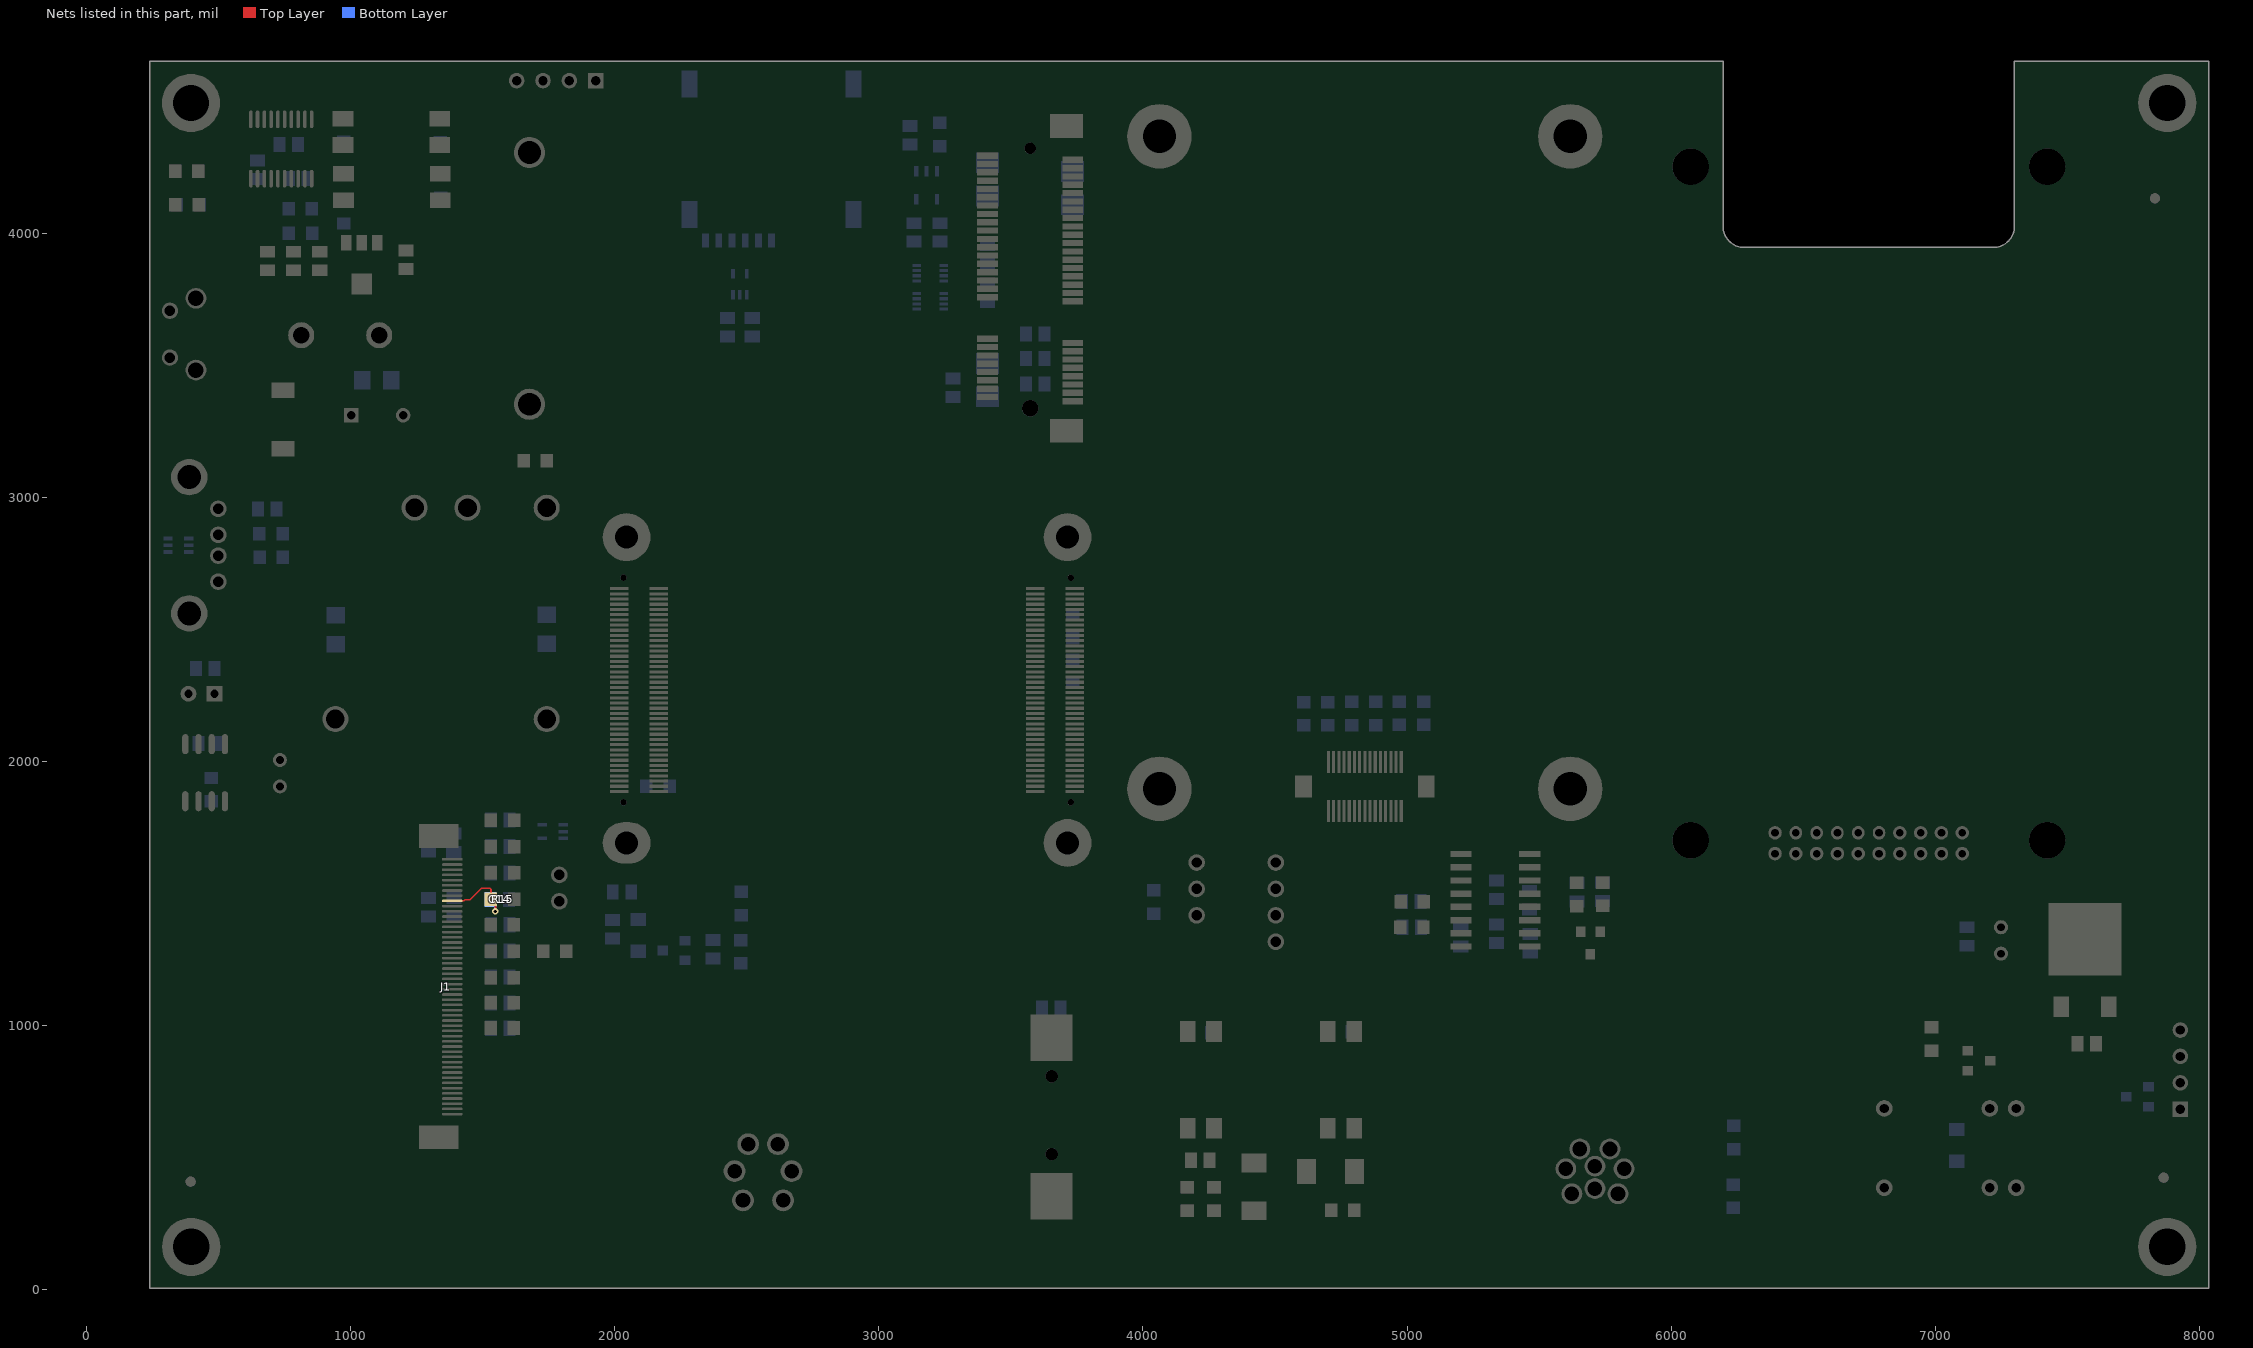
[diagram p0: the nets of this part, all layers, seen from the top]
# Altium PCB MISC82794.PcbDoc (part 5 of 5)
Units mil, origin at the board's own origin, x right, y up, seen from the top; angles counter-clockwise.
Board outline 7795.28 x 4645.67 mil, 4 copper layers (Top Layer, GND, POWER, Bottom Layer); 157 components, 133 nets, 768 pads, 456 vias.

## Via types
v1: diameter 24, hole 12, Top Layer to Bottom Layer, 258 vias
v2: diameter 40, hole 20, Top Layer to Bottom Layer, 197 vias
v3: diameter 30, hole 15, Top Layer to Bottom Layer, 1 vias

## Nets (pads, with @x,y where several pads share a name; then routed paths per layer and width w, separated by ;. In a path a pad name is that pad's centre, name@x,y a point inside that pad or via, vN(x,y) a via of type N, cw(c..) or ccw(c..) an arc to the next point about the centre after c; other vN are vias at no path point) (continued)
YP: C14.1 J1.9 R15.2 | length 313.2
  Top Layer w6: J1.9@1385.39,1472.65 1428.74,1472.65 1432.58,1476.49 1451.97,1476.49 1496.48,1521 1528,1521 1532,1517 R15.2@1532,1478.6 1549,1461.6 1549,1434 v1(1548,1433)
  Bottom Layer w6: C14.1@1531,1478.6 1547,1462.6 1547,1436 1549,1434 v1(1548,1433)
pads on no net: BT1.0 D5.1 D5.3 H1.8 H2.8 H3.8 H4.8 J1.10 J1.11 J1.13 J1.14 J1.15 J1.16 J1.18 J1.30 J1.31 J1.32 J1.40 J1.41 J1.48 J1.49 J1.50 J2.0 J2.1 J2.2 J2.3 J2.4 J2.A1 J2.A2 J2.A3 J2.A4 J2.A5 J2.A6 J2.A17 J2.A19 J2.A21 J2.A23 J2.A25 J2.A27 J2.A31 J2.A42 J2.A44 J2.A46 J2.A48 J2.A49 J2.A50 J2.A51 J2.A52 J2.A53 J2.A54 J2.A55 J2.A56 J2.A57 J2.A59 J2.A60 J2.A61 J2.A62 J2.A63 J2.A64 J2.A65 J2.A66 J2.A67 J2.A68 J2.A70 J2.A72 J2.A74 J2.A76 J2.A78 J2.A79 J2.A80 J2.B7 J2.B8 J2.B9 J2.B10 J2.B11 J2.B12 J2.B13 J2.B14 J2.B15 J2.B16 J2.B17 J2.B18 J2.B19 J2.B21 J2.B22 J2.B23 J2.B24 J2.B26 J2.B27 J2.B28 J2.B30 J2.B31 J2.B33 J2.B34 J2.B36 J2.B38 J2.B40 J2.B42 J2.B46 J2.B48 J2.B52 J2.B54 J2.B56 J2.B58 J2.B60 J2.B62 J2.B64 J2.B65 J2.B66 J2.B67 J2.B68 K1.3 K1.6 S1.3 S1.4 U6.0 U6.1 U6.3 U6.5 U6.6 U6.7 U6.11 U6.13 U6.16 U6.20 U6.23 U6.25 U6.28 U6.30 U6.31 U6.32 U6.33 U6.36 U6.38 U6.44 U6.45 U6.46 U6.47 U6.48 U6.49 U6.51 U6.53 U6.54 U9.3 U9.4 U9.7 U9.8 U9.20 U9.21 U9.22 U9.23 U9.24 U11.1 U11.2 U11.8 U13.1 U13.2 U13.3 U13.5 U13.6 U13.11 U13.12 U13.16 U13.17 U13.19 U13.20 U15.6 U15.10 U15.11 U17.0 U17.2 U17.4 U17.6 U17.8 U17.10 U17.12 U17.13 U17.15 U17.16 U17.17 U17.29 U17.31 U19.3 U19.6

## Polygon pours and split planes (outlines as drawn)
USB0_VBUS_5V on Bottom Layer "Top Layer-No Net" (solid, remove dead copper, pour order 1000): 1935.12,1937 1935.12,1914.88 1945,1905 1948,1902 1963,1902 1973,1902 1980,1909 1981,1910 1981,1925 1981,1934 1970,1945 1949,1945 1942.64,1945 1934.64,1937
VDD_12V on Bottom Layer "Top Layer-No Net" (solid, remove dead copper, pour order 1001): 4056,310.7 4056,257.46 4061,251.55 4064,248 4096,248 4189.74,248 4194,253.04 4198,257.77 4198,291.77 4198,321.35 4190,330.82 4189,332 4111,332 4067,332 4062,326.08 4056,318.99 4056,310.7
VDD_5V on Bottom Layer "Top Layer-No Net" (solid, remove dead copper, pour order 1002): 1239,1654 1239,1594 1248,1585 1253,1580 1274,1580 1311,1580 1321,1590 1362,1631 1390,1631 1416.66,1631 1420.66,1635 1425,1639.34 1425,1647 1425,1677.66 1420.66,1682 1419.66,1683 1412,1683 1244,1683 1239,1678 1239,1654
VDD_3.3 on Bottom Layer "Top Layer-No Net" (solid, remove dead copper, pour order 1003): 3075,4339 3075,4235 3091,4219 3097,4213 3131,4213 3150,4213 3153,4216 3156,4219 3156,4245 3156,4353 3150,4359 3148,4361 3128,4361 3082,4361 3075,4354 3075,4338
VDD_3.3 on Bottom Layer "Top Layer-No Net" (solid, remove dead copper, pour order 1004): 1237,1556 1237,1478 1249,1466 1256,1459 1278,1459 1424,1459 1428,1463 1431,1466 1431,1487 1431,1543 1405,1569 1401,1573 1309,1573 1246,1573 1237,1564 1237,1556
VDD_3.3 on Bottom Layer "Top Layer-No Net" (solid, remove dead copper, pour order 1005): 2895,1926 2895,1893 2901,1887 2907,1881 2928,1881 2932,1881 2934,1883 2936,1885 2936,1901 2936,1933 2933,1936 2931,1938 2924,1938 2902,1938 2898,1934 2895,1931 2895,1926
GND1 on Bottom Layer "Top Layer-No Net" (solid, remove dead copper, pour order 1006): 6200,638 6200,599 6204,595 6205,594 6240,594 6340,594 6348,602 6348,625 6348,656 6341,663 6335,669 6304,669 6207,669 6201,663 6200,662 6200,638
GND1 on Bottom Layer "Top Layer-No Net" (solid, remove dead copper, pour order 1007): 4227.2,303.17 4227.2,234.61 4234.4,229.37 4240.4,225 4270.4,225 4304,225 4312.4,231.12 4316,233.74 4316,259.96 4316,320.61 4309.28,325.5 4304.48,329 4281.2,329 4235.6,329 4228.4,323.76 4226,322.01 4226,303.17
GND on Bottom Layer "Top Layer-No Net" (solid, remove dead copper, pour order 1008): 61.25,4802.36 61.25,-271.65 -22.75,-355.65 228.25,-104.65 8117.25,-104.65 8117.25,4836.36 8251.25,4970.36 8132.25,4851.36 88.25,4851.36 88.25,4831.36 65.25,4808.36
GND1 on Top Layer "Top Layer-No Net" (solid, remove dead copper): 653,3873 653,3829 710,3772 750,3732 847,3732 903,3732 939,3696 943,3692 943,3650 943,3604 973,3574 993,3554 1074,3554 1097,3531 1149,3479 1149,3360 1149,3268 1159,3258 1166,3251 1190,3251 1276,3251 1288,3263 1295,3270 1295,3331 1295,3867 1276,3886 1273,3889 1244,3889 1082,3889 1075,3896 1069,3902 1069,3934 1069,3987 1062,3994 1059,3997 1051,3997 1023,3997 1021,3995 1019,3993 1019,3986 1019,3903 1015,3899 1002,3886 917,3886 659,3886 653,3880 653,3873
VDD_12V on Top Layer "Top Layer-No Net" (solid, remove dead copper): 268.85,3562.15 268.85,3508.15 268.85,3505.15 279.85,3494.15 334.85,3494.15 335.85,3494.15 390.85,3549.15 482.85,3549.15 509.85,3522.15 509.85,3508.15 509.85,3410.15 563.85,3356.15 778.85,3356.15 779.85,3356.15 890.85,3245.15 1023.85,3245.15 1041.85,3263.15 1042.85,3264.15 1042.85,3440.15 883.85,3599.15 883.85,3606.15 883.85,3664.15 836.85,3711.15 748.85,3711.15 743.85,3716.15 632.85,3827.15 632.85,3881.15 632.85,3894.15 640.85,3902.15 644.85,3906.15 671.85,3906.15 991.85,3906.15 1003.85,3918.15 1003.85,3942.15 1003.85,3997.15 999.85,4001.15 952.85,4001.15 793.85,4001.15 775.85,3983.15 760.85,3968.15 713.85,3968.15 568.85,3968.15 544.85,3944.15 527.85,3927.15 527.85,3906.15 527.85,3730.15 431.85,3634.15 429.85,3632.15 343.85,3632.15 324.85,3632.15 276.85,3584.15 268.85,3576.15 268.85,3562.15
USB0_VBUS_5V on Top Layer "Top Layer-No Net" (solid, remove dead copper, pour order 1009): 1935.12,1933 1935.12,1910.88 1940,1906 1946,1900 1960,1900 1968,1900 1979,1911 1986,1918 1995,1918 2055,1918 2056,1919 2057,1920 2057,1923 2057,1932 2055,1934 2054,1935 2049,1935 1977,1935 1970,1942 1967,1945 1957,1945 1942,1945 1938,1941 1935.12,1938.12 1935.12,1933
NetC4_1 on Top Layer "Top Layer-No Net" (solid, remove dead copper, pour order 1011): 647,3180 647,3080 647,3070 662,3055 668,3049 750,3049 1134,3049 1144,3039 1151,3032 1151,2997 1151,2925 1165,2911 1185,2891 1228,2891 1285,2891 1298,2904 1314,2920 1314,2958 1314,3107 1289,3132 1246,3175 1116,3175 895,3175 850,3220 843,3227 754,3227 669,3227 656,3214 647,3205 647,3178
VDD_5V on Top Layer "Top Layer-No Net" (solid, remove dead copper, pour order 1012): 805,2225 805,2190 805,2184 768,2147 760,2139 729,2139 700,2139 640,2079 549,1988 489,1988 463,1988 449,2002 442,2009 442,2037 442,2102 437,2107 436,2108 431,2108 413,2108 410,2105 407,2102 407,2094 407,1948 428,1927 431,1924 469,1924 611,1924 636,1949 663,1976 731,1976 909,1976 993,2060 1004,2071 1004,2180 1004,2234 994,2244 989,2249 975,2249 818,2249 805,2236 805,2225
VDD_12V on Top Layer "Top Layer-No Net" (solid, remove dead copper, pour order 1013): 4704,344 4624,344 4616,336 4614,334 4614,311 4614,273 4624,263 4626,261 4662,261 4732,261 4737,266 4744,273 4744,288 4744,334 4736,342 4734,344 4709,344
VDD_5V on Top Layer "Top Layer-No Net" (solid, remove dead copper, pour order 1014): 7582,944 7582,896 7590,888 7595,883 7628,883 7726,883 7732,889 7738,895 7738,960 7738,1116 7733,1121 7728,1126 7701,1126 7621,1126 7617,1122 7609,1114 7609,1103 7609,997 7597,985 7582,970 7582,944
VDD_5V on Top Layer "Top Layer-No Net" (solid, remove dead copper, pour order 1015): 3528,1905 3528,1879 3521,1872 3508,1859 3508,1826 3508,1790 3517,1781 3522,1776 3541,1776 3628,1776 3669,1817 3672,1820 3672,1839 3672,1859 3680,1867 3689,1876 3709,1876 3778,1876 3781,1879 3783,1881 3783,1887 3783,1910 3780,1913 3777,1913 3536,1913 3528,1905
VDD_3.3 on Top Layer "Top Layer-No Net" (solid, remove dead copper, pour order 1016): 7213,1418 7213,1354 7221,1346 7224,1343 7243,1343 7376,1343 7388,1331 7401,1318 7401,1288 7401,1210 7418,1193 7422,1189 7459,1189 7705,1189 7714,1198 7722,1206 7722,1242 7722,1482 7710,1494 7698,1506 7656,1506 7225,1506 7218,1499 7213,1494 7213,1418
VDD_5V on Top Layer "Top Layer-No Net" (solid, remove dead copper, pour order 1017): 1240,1623 1240,1596 1248,1588 1252,1584 1284,1584 1313,1584 1324,1595 1333,1604 1359,1604 1423,1604 1427,1608 1429,1610 1429,1622 1429,1635 1426,1638 1424,1640 1416,1640 1247,1640 1240,1633 1240,1623
VDD_3.3 on Top Layer "Top Layer-No Net" (solid, remove dead copper, pour order 1018): 1419,1577 1309,1577 1254,1577 1249,1572 1243,1566 1243,1558 1243,1537 1248,1532 1251,1529 1275,1529 1316,1529 1326,1539 1332,1545 1356,1545 1427,1545 1429,1547 1431,1549 1431,1557 1431,1573 1427,1577 1419,1577
GND1 on Top Layer "Top Layer-No Net" (solid, remove dead copper, pour order 1019): 4363,577 4363,452 4373,442 4377,438 4404,438 4487,438 4522,403 4533,392 4584,392 4656,392 4659,395 4664,400 4664,417 4664,491 4725,552 4732,559 4732,586 4732,650 4729,653 4728,654 4721,654 4397,654 4383,640 4363,620 4363,577
GND on Top Layer "Top Layer-No Net" (solid, remove dead copper, pour order 1021): 36.44,4726.77 36.44,-163.23 106.44,-233.23 137.44,-264.23 8137.44,-264.23 8137.44,4781.77 8160.44,4804.77 8082.44,4726.77 36.44,4726.77
GND on GND (split plane): 205 vertices, not listed, extent 259.65,25.91 8014.74,4631.39
GND1 on GND (split plane): 1570.91,3981.4 1570.91,1959.6 1178.66,1567.34 1175.2,1563.4 1172.28,1559.04 1169.97,1554.34 1168.28,1549.38 1167.26,1544.23 1166.91,1539 1166.91,541 1167.26,535.77 1168.28,530.62 1169.97,525.66 1172.28,520.96 1175.2,516.6 1178.66,512.66 1271.66,419.65 1275.6,416.2 1279.96,413.28 1284.66,410.97 1289.62,409.28 1294.77,408.26 1300,407.91 1638,407.91 1643.23,408.26 1648.38,409.28 1653.34,410.97 1658.04,413.28 1662.4,416.2 1666.34,419.66 2136.6,889.91 4265,889.91 4270.23,890.26 4275.38,891.28 4280.34,892.97 4285.04,895.28 4289.4,898.2 4293.34,901.66 4370.34,978.65 4373.8,982.6 4376.72,986.96 4379.03,991.66 4380.72,996.62 4381.74,1001.77 4382.09,1007 4382.09,1135 4381.74,1140.23 4380.72,1145.38 4379.03,1150.34 4376.72,1155.04 4373.8,1159.4 4370.34,1163.34 4123.09,1410.6 4123.09,1612.4 4185.6,1674.91 4322.4,1674.91 4398.91,1598.4 4398.91,1427 4399.26,1421.77 4400.28,1416.62 4401.97,1411.66 4404.28,1406.96 4407.2,1402.6 4410.66,1398.66 4693.65,1115.66 4697.6,1112.2 4701.96,1109.28 4706.66,1106.97 4711.62,1105.28 4716.77,1104.26 4722,1103.91 6280.4,1103.91 6429.91,954.4 6429.91,25.91 259.65,25.91 259.65,3325.93 463.9,3121.68 463.9,3031.32 402.79,2970.21 400.29,2967.17 398.43,2963.69 397.29,2959.92 396.9,2956 396.9,2675 397.29,2671.08 398.43,2667.31 400.29,2663.83 402.79,2660.79 453.9,2609.68 453.9,2504.32 329.79,2380.21 327.29,2377.17 325.43,2373.69 324.29,2369.92 323.9,2366 323.9,1988 324.29,1984.08 325.43,1980.31 327.29,1976.83 329.79,1973.79 448.27,1855.31 447.26,1850.23 446.91,1845 447.26,1839.77 448.28,1834.62 449.97,1829.66 452.28,1824.96 455.2,1820.6 458.66,1816.66 462.6,1813.2 466.96,1810.28 471.66,1807.97 476.62,1806.28 481.77,1805.26 487,1804.91 783,1804.91 788.23,1805.26 793.38,1806.28 798.34,1807.97 803.04,1810.28 807.4,1813.2 811.34,1816.66 857.34,1862.65 860.8,1866.6 863.72,1870.96 866.03,1875.66 867.72,1880.62 868.74,1885.77 869.09,1891 869.09,3166 868.74,3171.23 867.72,3176.37 866.03,3181.34 863.72,3186.04 860.8,3190.4 857.34,3194.34 636.09,3415.6 636.09,4430.4 686.6,4480.91 1071.4,4480.91
VDD_3.3 on POWER (split plane): 264 vertices, not listed, extent 259.65,1160.09 8014.74,4631.39
VDD_12V on POWER (split plane): 263,3669.91 841.4,3669.91 1046.91,3464.4 1046.91,3292.6 822.66,3068.34 819.2,3064.4 816.28,3060.04 813.97,3055.34 812.28,3050.37 811.26,3045.23 810.91,3040 810.91,1076 811.26,1070.77 812.28,1065.62 813.97,1060.66 816.28,1055.96 819.2,1051.6 822.66,1047.66 1235.66,634.66 1239.6,631.2 1243.96,628.28 1248.66,625.97 1253.62,624.28 1258.77,623.26 1264,622.91 6775.4,622.91 6897.91,500.4 6897.91,30 6898.18,25.91 259.65,25.91 259.65,3670.13
VDD_5V on POWER (split plane): 188 vertices, not listed, extent 891.09,25.91 8014.74,2273.91

## Keep-outs
Keep-Out Layer:
  lines w5: 239.55,5.82 8034.83,5.82 8034.83,4651.49 7298.61,4651.49 7298.61,4025.5 cw(c7219.87,4025.5) 7219.87,3946.76 6274.99,3946.76 cw(c6274.99,4025.5) 6196.25,4025.5 6196.25,4651.49 239.55,4651.49 239.55,3765.66 239.55,2559.75 239.55,5.82

## Other copper
GND (plane layer: these items are gaps in the copper):
  lines w30: 596,3399 596,3412
  lines w40: 254,3360 484,3130 484,3023 417,2956 417,2675 474,2618 474,2496 344,2366 344,1988 487,1845
  lines w80: 487,1845 783,1845 829,1891 829,3166 596,3399 ; 596,3412 596,4447 670,4521 1088,4521 1611,3998 1611,1943 1207,1539 1207,541 1300,448 1638,448 2120,930 2301,930 4265,930 4342,1007 4342,1135 4083,1394 4083,1629 4169,1715 4339,1715 4439,1615 4439,1427 4722,1144 6297,1144 6470,971 6470,8
POWER (plane layer: these items are gaps in the copper):
  lines w20: 1269.32,1477.68 1226,1521 1226,1563 1241,1578 1333,1578 ; 6184,1421 6202,1421 ; 6844,1695 7130,1695 7161,1664
  lines w40: 1333,1578 1456.43,1701.43
  lines w80: 263,3710 858,3710 1087,3481 1087,3276 851,3040 851,1076 1264,663 6792,663 6938,517 6938,30 ; 860,2314 1318,2314 ; 1272,1475 1588,1475 1757,1644 1856,1644 1926,1574 1926,1272 2078,1120 2610,1120 2843,1353 2843,1674 3096,1927 3744,1927 3843,1828 3843,1535 4061,1317 4554,1317 4639,1402 4980,1402 5223,1159 5922,1159 6184,1421 ; 1320.83,2311.17 1456.43,2175.57 1456.43,1934.43 ; 1456.43,1701.43 1456.43,1938 ; 6202,1421 6570,1421 6844,1695 ; 7161,1664 7161,1594 6972,1405 6972,1225 7042,1155 8013,1155

## Silkscreen, mask and mechanical layers (free items; w line width, h text height)
Top Overlay:
  lines w6: 1708,1696 1773,1696 ; 1749,1699 1782,1666 1782,1665 ; 1778,1664 1779,1664 1814,1699
  lines w12.2: 5555.45,67.05 cw(c5709.72,-9.51) 5863,69
  text "GND1" at 2022,4471 h45
  text "SWIM" at 1477,4468 h45
  text "RESET" at 1671,4468 h45
  text "5V" at 1915,4467 h45
  text "GND" at 7737,966 h45
  text "5V" at 7770,860 h45
  text "TX1" at 7749,759 h45
  text "RX1" at 7743,655 h45
  text "Nav_Board" at 824,316 h45
  text "Ver:3.0" at 849,206 h45
  text "2018-06-10" at 807,100 h45
Mechanical 2:
  circle w5: c5712,438.89 r314.96
  circle w5: c2562.39,438.89 r314.96
  circle w5: c397.03,4494.01 r68.9
  circle w5: c7877.35,4494.01 r68.9
  circle w5: c7877.35,163.3 r68.9
  circle w5: c397.03,163.3 r68.9
  lines w5: 239.55,3549.12 28.92,3549.12 28.92,3686.92 239.55,3686.92 ; 5715.48,1235.35 5729.66,1235.35 ; 3.33,2559.75 3.33,3076.68 554.51,3076.68 554.51,2559.75 3.33,2559.75 ; 239.55,3470.38 239.55,3765.66 383.25,3765.66 383.25,3470.38 239.55,3470.38
  text "USB" at 10277.86,2822.86 h45
Mechanical 4:
  circle w5: c5712,438.89 r399.61
  circle w5: c2562.39,438.89 r399.61
  lines w5: 600.86,1821 611,1821 611,1820.88 1879.83,1820.88 1879.83,3074.54 1327.02,3074.54 1327.02,4497.12 600.86,4497.12 600.86,1821 ; 1184.44,557 1184.44,1738.1 1420.66,1738.1 1420.66,557 1184.44,557 ; 1379.16,3160.87 3820.11,3160.87 3820.11,4499.45 1379.16,4499.45 1379.16,3160.87 ; 1474.83,1356.96 1474.83,1797.44 1934.64,1797.44 1934.64,1356.96 1474.83,1356.96 ; 1696.25,5.82 1696.25,1186.92 6578.14,1186.92 6578.14,5.82 1696.25,5.82 ; 1934.64,1581.85 3824.4,1581.85 3824.4,2959.8 1934.64,2959.8 1934.64,1581.85 ; 3924.07,1752.45 3924.07,4508.36 5759.11,4508.36 5759.11,1752.45 3924.07,1752.45 ; 5841.92,1584.56 5841.92,4379.83 7652.94,4379.83 7652.94,1584.56 5841.92,1584.56 ; 6628.61,294.91 6628.61,1515.66 7951.5,1515.66 7951.5,294.91 6628.61,294.91
Mechanical 8:
  circle w7.87: c5467.44,432.17 r314.96
  circle w7.87: c2317.84,432.17 r314.96
  circle w7.87: c152.48,156.58 r68.9
  circle w7.87: c7632.8,156.58 r68.9
  circle w7.87: c152.48,4487.29 r68.9
  circle w7.87: c7632.8,4487.29 r68.9
  circle w7.87: c2317.84,432.17 r399.61
  circle w7.87: c5467.44,432.17 r399.61
  lines w7.87: -5,3542.41 -215.63,3542.41 -215.63,3680.2 -5,3680.2 ; 309.96,2553.04 -241.22,2553.04 -241.22,3069.97 309.96,3069.97 ; 331.96,2558.04 331.96,3074.97 ; 939.88,1731.38 939.88,550.28 1176.1,550.28 1176.1,1731.38 ; 965.88,1729.38 1202.1,1729.38 ; -5,3463.67 -5,3758.94 138.7,3758.94 138.7,3463.67 -5,3463.67 ; 703.66,2443.98 703.66,4333.75 2081.62,4333.75 2081.62,2443.98 703.66,2443.98 ; 1451.69,-0.9 6333.59,-0.9 6333.59,1180.2 1451.69,1180.2 1451.69,-0.9 ; 1950.99,1309.32 5166.32,1309.32 5166.32,2292.22 1950.99,2292.22 1950.99,1309.32 ; 2120.99,2443.98 4561.93,2443.98 4561.93,3782.57 2120.99,3782.57 2120.99,2443.98 ; 4601.3,2443.98 4601.3,4136.9 5546.18,4136.9 5546.18,2443.98 4601.3,2443.98 ; 5597.37,1577.84 7408.39,1577.84 7408.39,4373.12 5597.37,4373.12 5597.37,1577.84